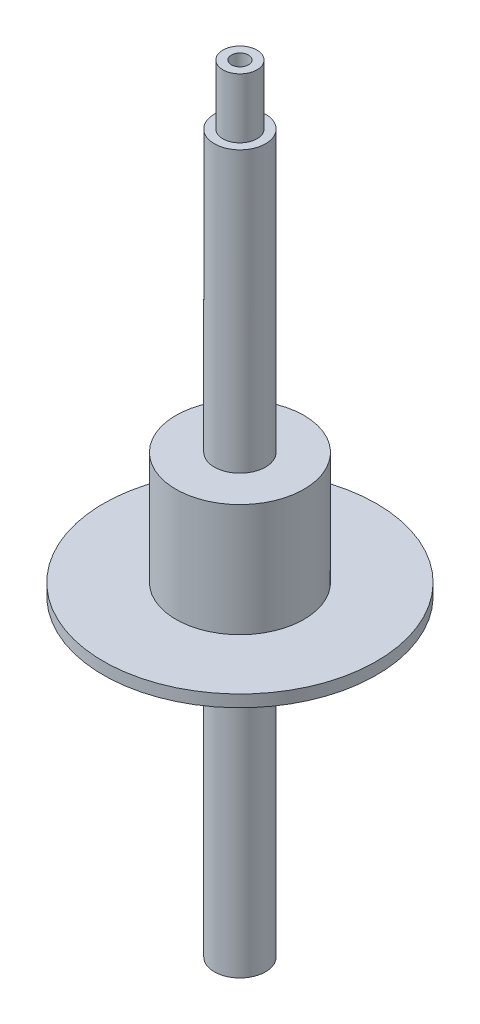
SolidWorks part; units mm, degrees
ref_plane "Front Plane" through (0, 0, 0) normal (0, 0, 1) x (1, 0, 0)
ref_plane "Top Plane" through (0, 0, 0) normal (0, 1, 0) x (1, 0, 0)
ref_plane "Right Plane" through (0, 0, 0) normal (1, 0, 0) x (0, 0, -1)
sketch "Sketch1" plane through (0, 0, 0) normal (0, 0, 1) x (1, 0, 0)
  line L0 (0, 0) -> (0, 49.8148) construction
  line L1 (0, 0) -> (1.5, 0)
  line L2 (1.5, 0) -> (1.5, 18.3)
  line L3 (1.5, 18.3) -> (8, 18.3)
  line L4 (8, 18.3) -> (8, 19)
  line L5 (8, 19) -> (3.75, 19)
  line L6 (3.75, 19) -> (3.75, 25.6)
  line L7 (3.75, 25.6) -> (1.5, 25.6)
  line L8 (1.5, 25.6) -> (1.5, 45.5)
  line L9 (1.5, 45.5) -> (0, 45.5)
  line L10 (0, 45.5) -> (0, 0)
  dimension "D1" = 3
  dimension "D2" = 45.5
  dimension "D3" = 16
  dimension "D4" = 0.7
  dimension "D5" = 7.5
  dimension "D6" = 7.3
  dimension "D7" = 18.3
revolve "Revolve1" add sketch "Sketch1" angle 360 about L0
sketch "Sketch3" plane through (0, 0, 0) normal (0, -1, 0) x (1, 0, 0)
  circle A0 centre (0, 0) radius 0.5
  dimension "D1" = 1
extrude "Cut-Extrude1" cut sketch "Sketch3" against normal through all
sketch "Sketch4" plane through (0, 45.5, 0) normal (0, 1, 0) x (1, 0, 0)
  circle A0 centre (0, 0) radius 1
  dimension "D1" = 2
extrude "Cut-Extrude2" cut sketch "Sketch4" against normal blind 3.5 flip side to cut
